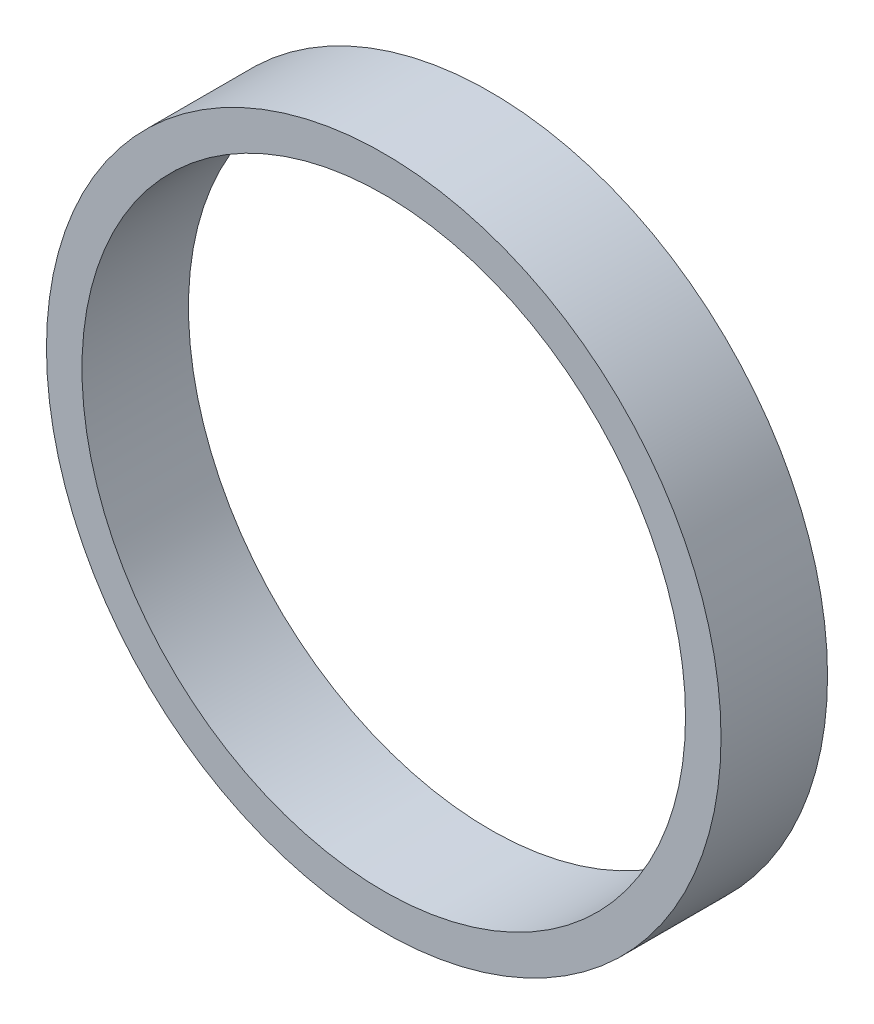
from build123d import *

# Parameters (mm, degrees)
SKETCH2_R           = 95
SKETCH2_R_2         = 85
BOSS_EXTRUDE1_DEPTH = 30


with BuildPart() as part:
    # Sketch2 → Boss-Extrude1 (new body)
    with BuildSketch(Plane.XY):
        Circle(SKETCH2_R)
        Circle(SKETCH2_R_2, mode=Mode.SUBTRACT)
    extrude(amount=BOSS_EXTRUDE1_DEPTH)


solid = part.part
